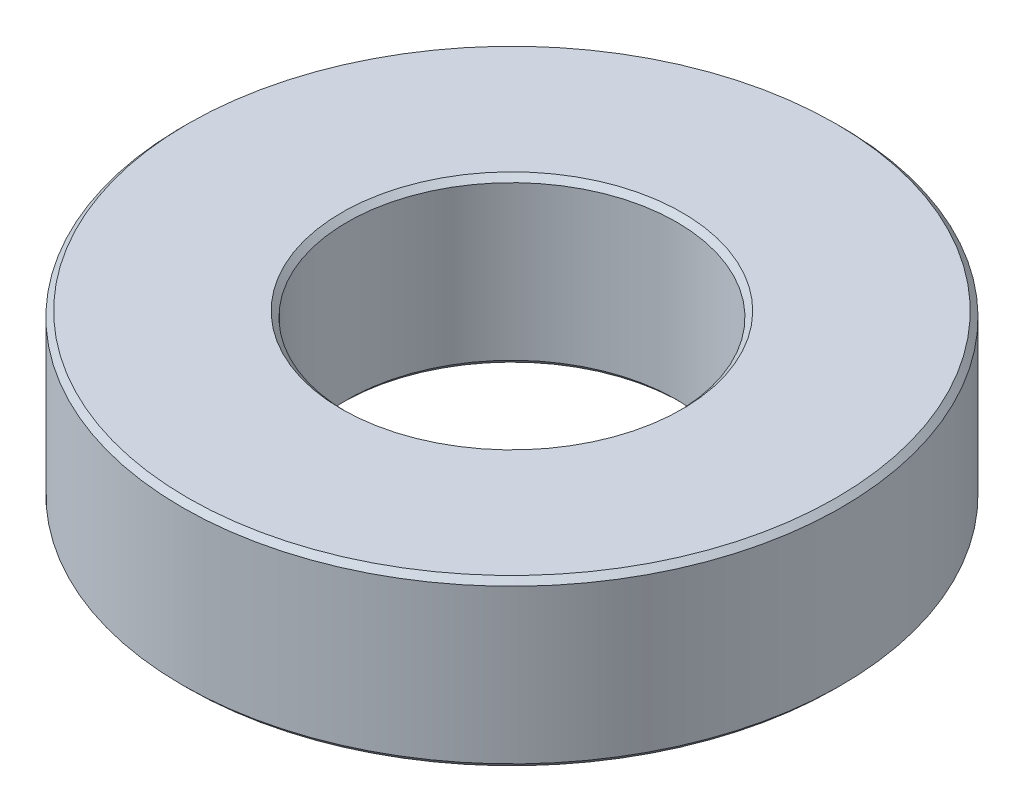
SolidWorks part; units mm, degrees
ref_plane "前视基准面" through (0, 0, 0) normal (0, 0, 1) x (1, 0, 0)
ref_plane "上视基准面" through (0, 0, 0) normal (0, 1, 0) x (1, 0, 0)
ref_plane "右视基准面" through (0, 0, 0) normal (1, 0, 0) x (0, 0, -1)
sketch "草图1" plane through (0, 0, 0) normal (0, 1, 0) x (1, 0, 0)
  circle A0 centre (0, 0) radius 12
  circle A1 centre (0, 0) radius 6
extrude "拉伸1" add sketch "草图1" along normal blind 6
chamfer "倒角1" distance 0.2 angle 45 4 edges at (0, 0, 12) (0, 0, 6) (0, 6, 12) (0, 6, 6)
